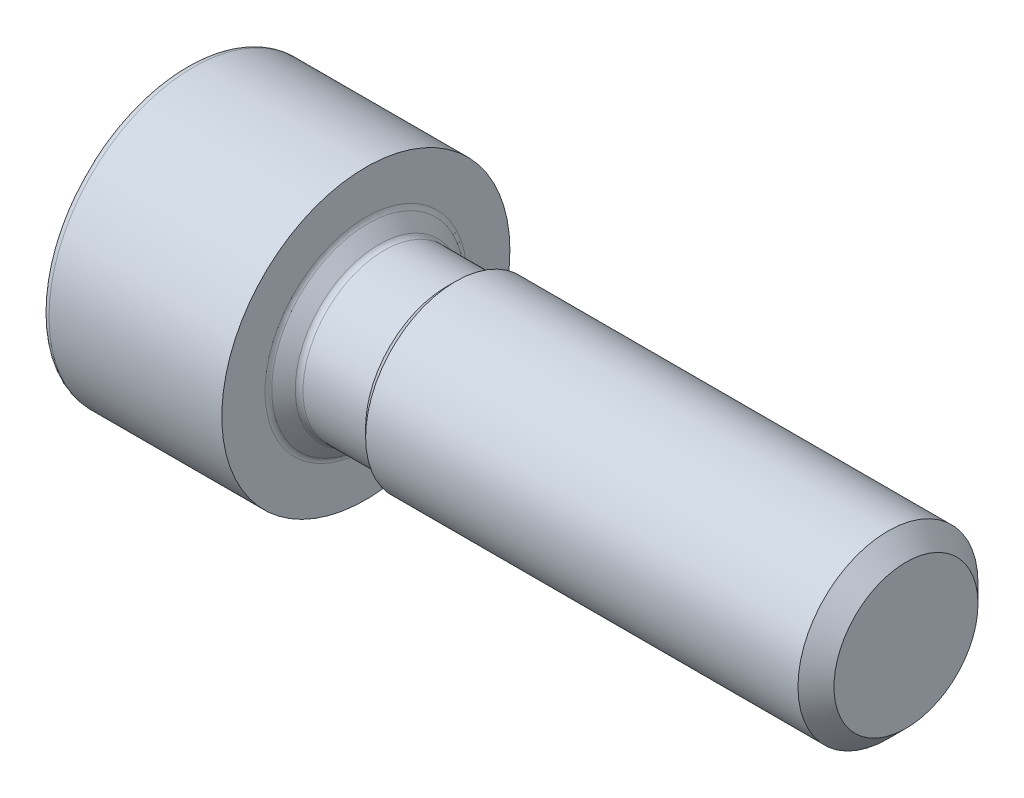
SolidWorks part; units mm, degrees
ref_plane "Front Plane" through (0, 0, 0) normal (0, 0, 1) x (1, 0, 0)
ref_plane "Top Plane" through (0, 0, 0) normal (0, 1, 0) x (1, 0, 0)
ref_plane "Right Plane" through (0, 0, 0) normal (1, 0, 0) x (0, 0, -1)
sketch "Dimension Sketch" plane through (0, 0, 0) normal (0, 0, 1) x (1, 0, 0)
  line L0 (0, 0) -> (40, 0) construction
  point P2 (11.2, 0)
  point P3 (30.85, 0)
  point P4 (38.5, 0)
  point P5 (5, 0)
  point P6 (16, 0)
  point P7 (10, 0)
  point P8 (10, 0)
  point P9 (25.026, 0)
  point P10 (26.046, 0)
  point P11 (0.4, 0)
  point P12 (8, 0)
  point P14 (22.85, 0)
  point P15 (27.046, 0)
  point P16 (0, 15.33)
  point P17 (0, 11.33)
  dimension "k" = 10
  dimension "l" = 30
  dimension "t" = 5
  dimension "dk" = 16
  dimension "d" = 10
  dimension "da" = 11.2
  dimension "b" = 32
  dimension "e" = 9.15
  dimension "p" = 1.5
  dimension "ds" = 9.026
  dimension "lf" = 1.02
  dimension "r" = 0.4
  dimension "s" = 8
  dimension "v" = 1
  dimension "dw" = 15.33
  dimension "w" = 4
sketch "Sketch1" plane through (0, 0, 0) normal (0, 0, 1) x (1, 0, 0)
  line L1 (0, 0) -> (0, 8)
  line L2 (0, 8) -> (10, 8)
  line L3 (10, 8) -> (10, 5.6)
  line L4 (11.02, 4.513) -> (14.5, 4.513)
  line L5 (40, 5) -> (40, 0)
  line L6 (0, 0) -> (40, 0)
  line L7 (0, 0) -> (-33.993, 0) construction
  line L8 (10.103, 5.332) -> (10.723, 4.645)
  line L9 (14.5, 4.513) -> (14.987, 5)
  line L10 (14.987, 5) -> (40, 5)
  line L11 (8.6414, 0) -> (6, 4.575) construction
  line L12 (6, 4.575) -> (0, 4.575) construction
  line L13 (8.6414, 0) -> (6, -4.575) construction
  line L14 (6, -4.575) -> (0, -4.575) construction
  arc A0 (11.02, 4.513) -> (10.723, 4.645) centre (11.02, 4.913) cw
  arc A1 (10.103, 5.332) -> (10, 5.6) centre (10.4, 5.6) cw
  point P10 (6, 8)
  point P21 (0.634, 8)
  dimension "D1" = 0.4
  dimension "D2" = 10
  dimension "dk" = 16
  dimension "D3" = 10
  dimension "l" = 30
  dimension "D5" = 45
  dimension "da" = 11.2
  dimension "lt" = 1.02
  dimension "ds" = 9.026
  dimension "ls" = 4.5
  dimension "D6" = 120
  dimension "w" = 4
  dimension "D7" = 9.15
  dimension "f" = 0.634
revolve "Base-Revolve" add sketch "Sketch1" angle 360 about L7
cosmetic thread "Cosmetic Thread1" parameters "D1"=25.5, "D2"=8.3763
sketch "Sketch2" plane through (0, 0, 0) normal (-1, 0, 0) x (0, 0, 1)
  line L1 (3.9621, -2.2875) -> (3.9621, 2.2875)
  line L2 (3.9621, 2.2875) -> (0, 4.575)
  line L3 (0, 4.575) -> (-3.9621, 2.2875)
  line L4 (-3.9621, 2.2875) -> (-3.9621, -2.2875)
  line L5 (-3.9621, -2.2875) -> (0, -4.575)
  line L6 (0, -4.575) -> (3.9621, -2.2875)
  circle A0 centre (0, 0) radius 3.9621 construction
  dimension "e" = 9.15
extrude "Cut-Extrude1" cut sketch "Sketch2" against normal up to vertex (6 mm away) up to point (6, 4.575, 0)
ref_plane "Plane1" through (8.6414, 0, 0) normal (1, 0, 0) x (0, 0, -1)
sketch "Sketch13" plane through (0, 0, 0) normal (0, 0, 1) x (1, 0, 0)
  line L0 (0, 4.575) -> (0.6129, 3.9621)
  line L1 (0.6129, 3.9621) -> (0, 3.9621)
  line L2 (0, 0) -> (0, 8) construction
  line L3 (0, 3.9621) -> (0, 4.575)
  line L6 (0, 0) -> (-33.993, 0) construction
  line L7 (0, 0) -> (-33.993, 0) construction
  line L8 (6, 4.575) -> (0, 4.575) construction
  line L9 (6, 4.575) -> (0, 4.575) construction
  line L10 (3, 4.575) -> (3, 0) construction
  line L11 (0, 0) -> (40, 0) construction
  line L12 (6, 3.9621) -> (6, 4.575) construction
  line L13 (5.3871, 3.9621) -> (6, 3.9621) construction
  line L14 (6, 4.575) -> (5.3871, 3.9621) construction
  dimension "D1" = 45
revolve "Cut-Revolve4" cut sketch "Sketch13" angle 360 mid plane about L7
sketch "Sketch16" plane through (0, 0, 0) normal (0, 0, 1) x (1, 0, 0)
  line L0 (8.6414, 0) -> (6, 4.575) construction
  line L1 (0, 0) -> (40, 0) construction
  line L2 (8.6414, 0) -> (6, 4.575)
  line L3 (6, 0) -> (8.6414, 0)
  line L4 (6, 4.575) -> (6, 0)
revolve "Cut-Revolve5" cut sketch "Sketch16" angle 360 mid plane about L3
fillet "Fillet1" radius 0.4 1 edges at (0, 0, -8)
sketch "Sketch11" plane through (0, 0, 0) normal (0, 0, 1) x (1, 0, 0)
  line L0 (11.02, 4.76) -> (11.02, 9)
  line L1 (11.02, 9) -> (13.02, 9)
  line L2 (13.02, 9) -> (13.02, 4.76)
  line L3 (13.02, 4.76) -> (11.02, 4.76)
  line L4 (0, 0) -> (40, 0) construction
  line L5 (0, 0) -> (40, 0) construction
  dimension "垫圈d" = 9.52
  dimension "h" = 2
  dimension "d2" = 18
revolve "Revolve1" [suppressed] add sketch "Sketch11" angle 360 mid plane about L5
chamfer "Chamfer1" distance 1 angle 45 1 edges at (40, 0, -5)
